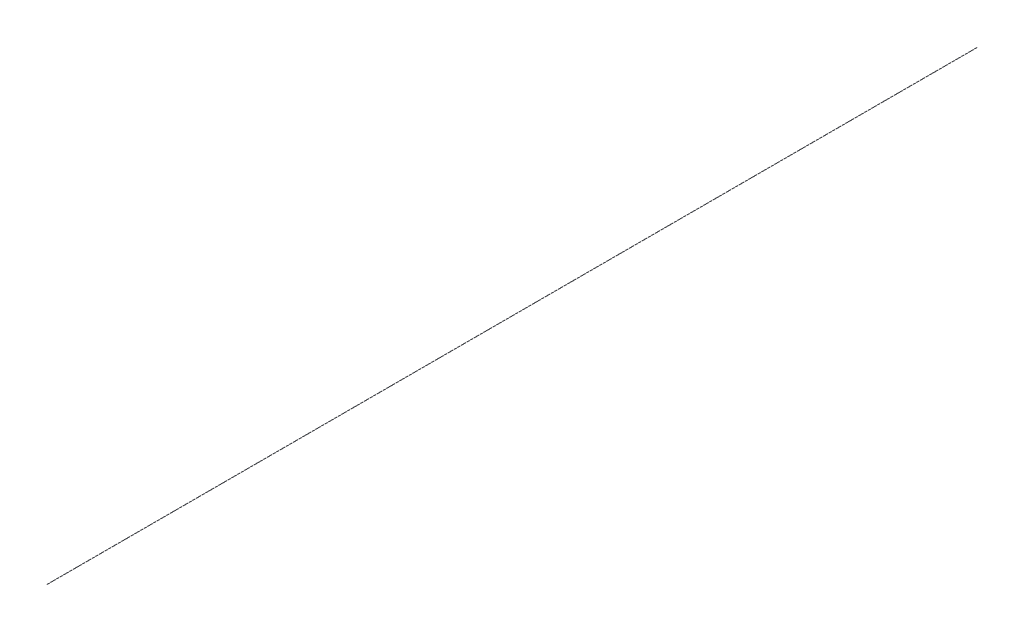
from build123d import *

# Parameters (mm, degrees)
SKETCH1_R           = 0.15
SKETCH1_R_2         = 0.075
BOSS_EXTRUDE1_DEPTH = 1900


with BuildPart() as part:
    # Sketch1 → Boss-Extrude1 (new body)
    with BuildSketch(Plane.XY):
        Circle(SKETCH1_R)
        Circle(SKETCH1_R_2, mode=Mode.SUBTRACT)
    extrude(amount=BOSS_EXTRUDE1_DEPTH)


solid = part.part
